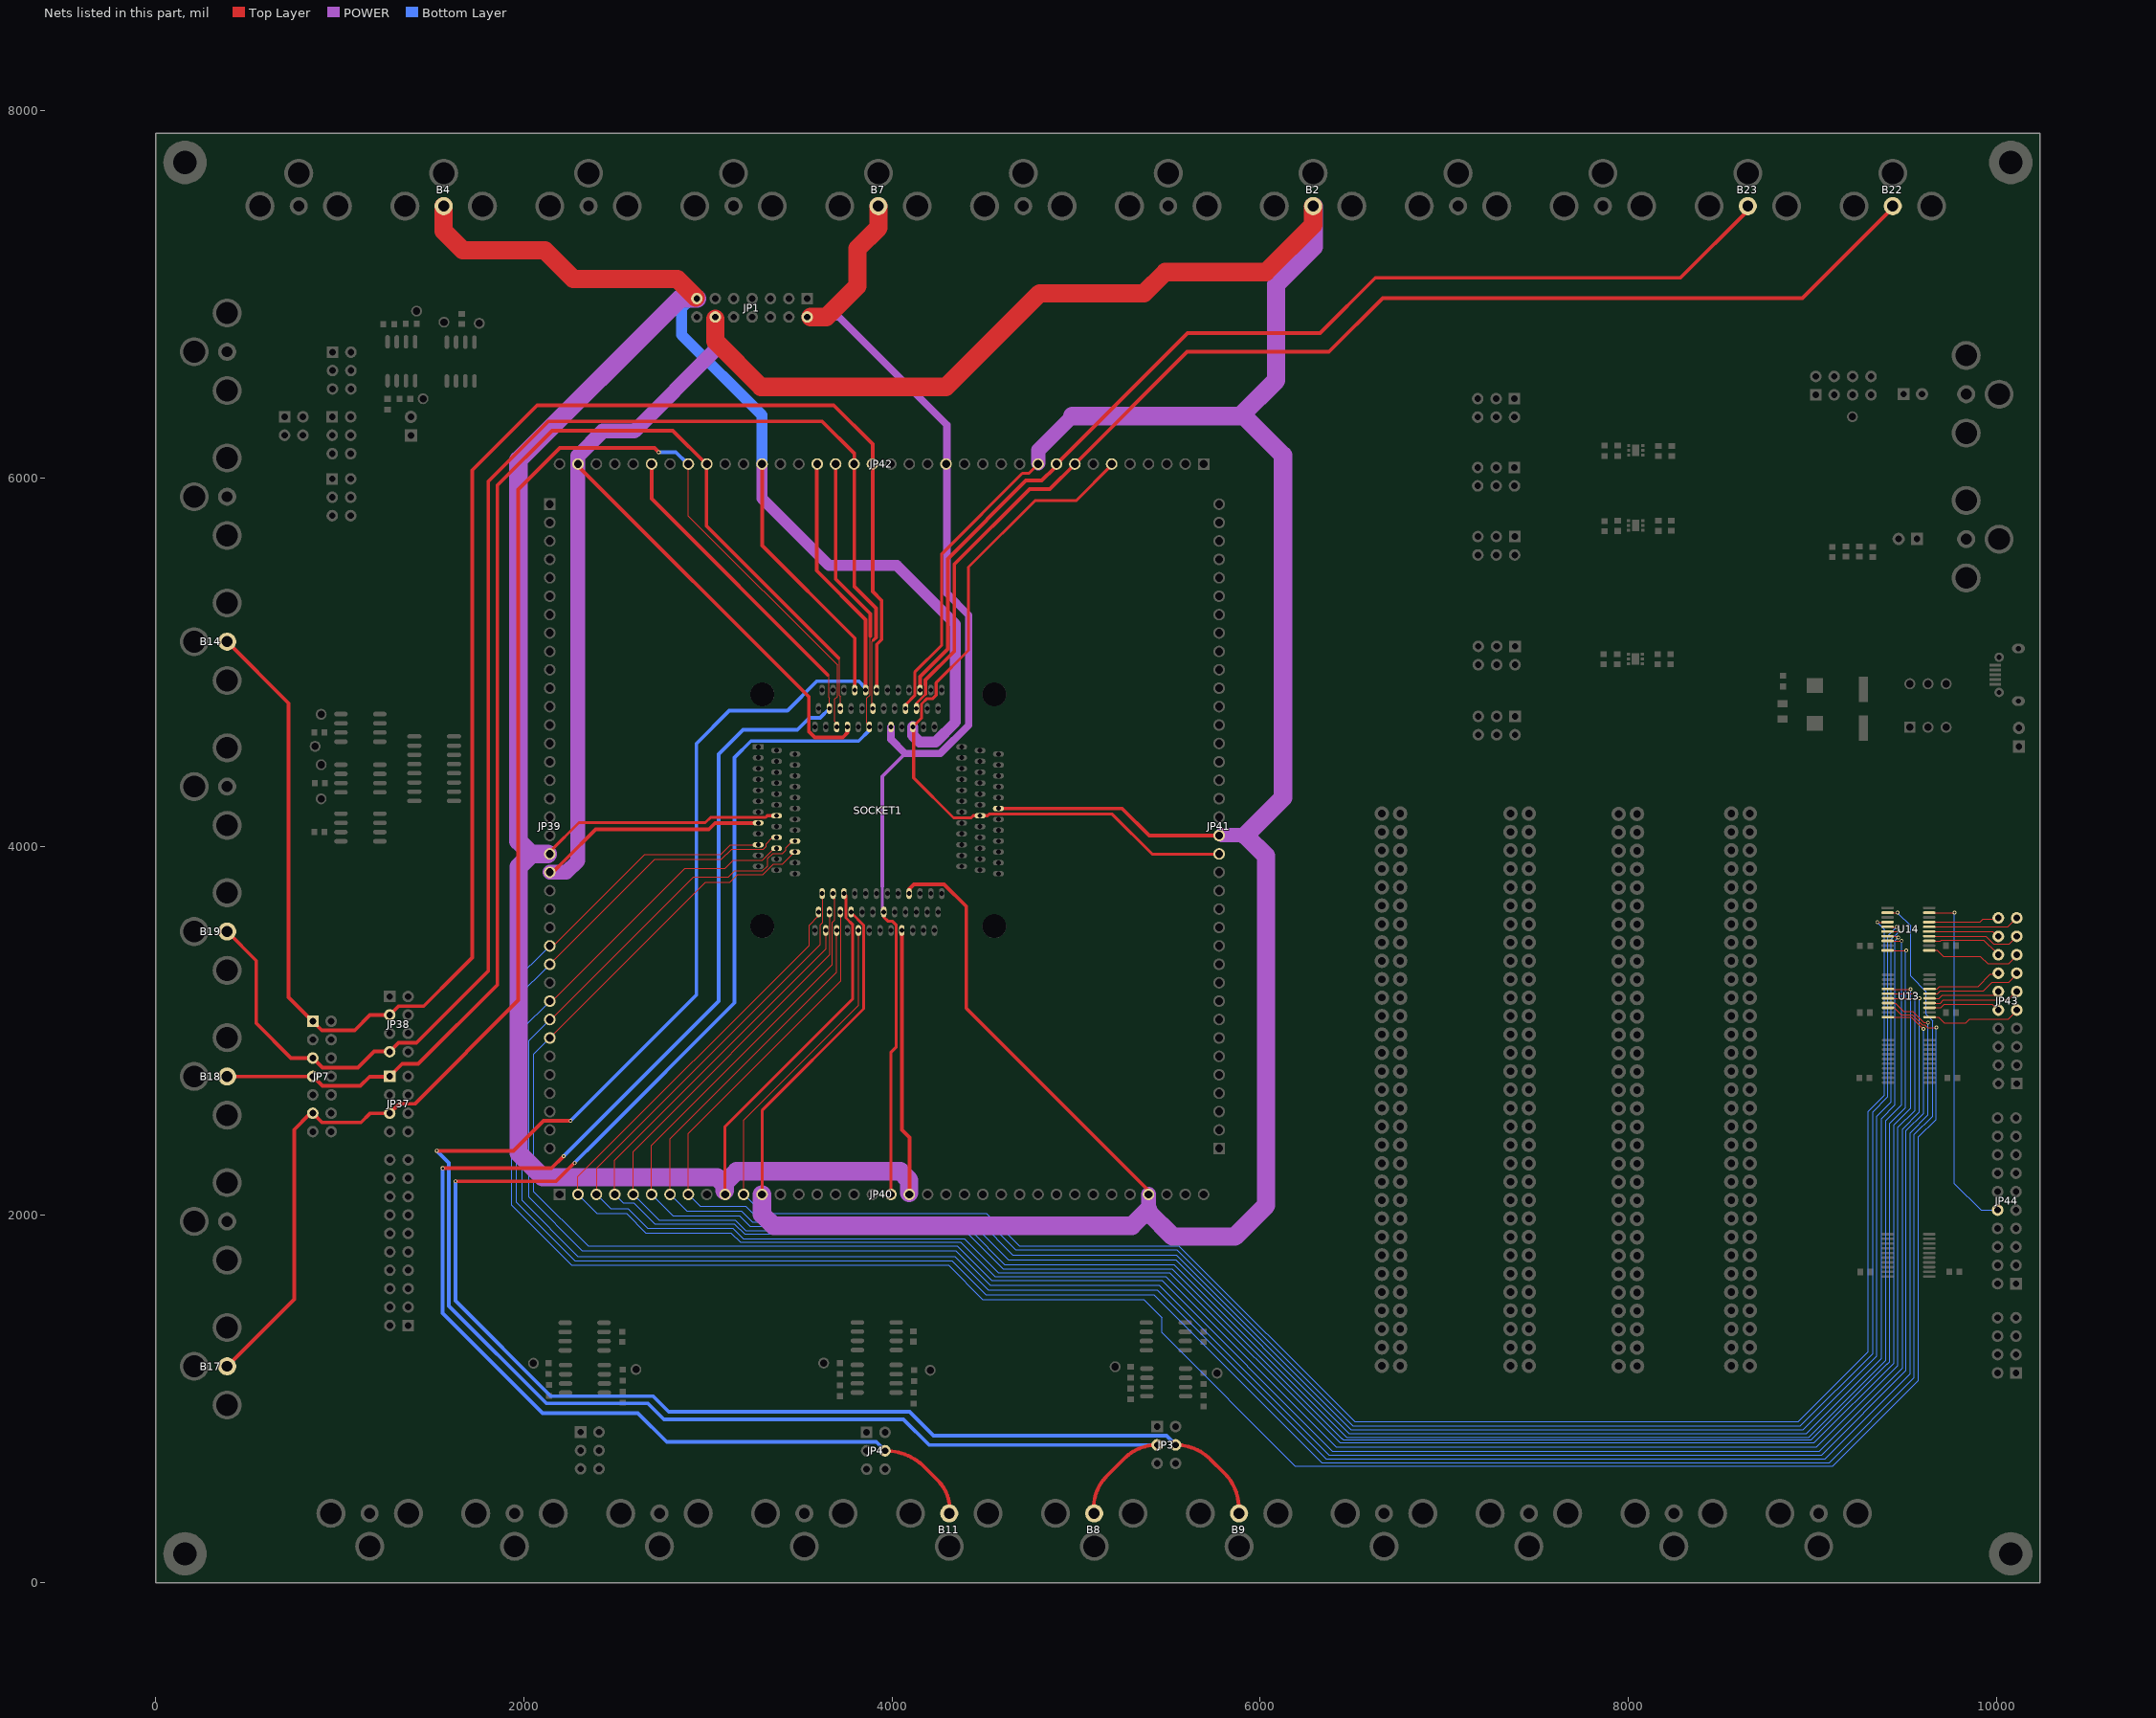
[diagram p0: the nets of this part, all layers, seen from the top]
# Altium PCB MISC62794.PcbDoc (part 6 of 7)
Units mil, origin at the board's own origin, x right, y up, seen from the top; angles counter-clockwise.
Board outline 10236.22 x 7874.02 mil, 4 copper layers (Top Layer, GND, POWER, Bottom Layer); 158 components, 185 nets, 1211 pads, 1759 vias.

## Via types
v1: diameter 20, hole 12, Top Layer to Bottom Layer, 1759 vias

## Nets (pads, with @x,y where several pads share a name; then routed paths per layer and width w, separated by ;. In a path a pad name is that pad's centre, name@x,y a point inside that pad or via, vN(x,y) a via of type N, cw(c..) or ccw(c..) an arc to the next point about the centre after c; other vN are vias at no path point) (continued)
VG2: B11.1 JP4.4 JP42.31 SOCKET1.140 | length 9670.1
  Top Layer w6: 3649.5,4934.5 3655.57,4928.43 3655.57,4809.69 3659.25,4806 SOCKET1.140@3659.25,4749.77
  Top Layer w20: v1(1558,2252) 2149,2252 v1(2215,2318) ; JP42.31@2693,6078.02 2693,5890 3649,4934 ; JP4.4@3961.48,717.38 cw(c3961.48,412.85) 4176.82,628.18 4246.12,558.88 cw(c4082.24,395) B11.1@4314,395
  Bottom Layer w20: v1(1558,2252) 1558,1464 2101,921 2619,921 2775.13,764.87 3913.98,764.87 JP4.4@3961.48,717.38 ; v1(2215,2318) 2371.5,2474.5 3057,3160 3057,4501 3190,4634 3485,4634 3550,4699 3608.48,4699 SOCKET1.140@3659.25,4749.77
VG_PS_CTRL: B17.1 JP7.11 JP37.5 JP42.29 SOCKET1.138 | length 8512
  Top Layer w6: JP42.29@2893,6058 2893,5796 3702.31,4986.69 3702.31,4815.31 3688,4801 3688,4679 SOCKET1.138@3696,4671
  Top Layer w20: B17.1@386.77,1176.09 751,1540.31 751,2462 JP7.11@835,2546 ; JP7.11@852,2551 902,2501 1114,2501 1163,2550 JP37.5@1253,2550 ; JP37.5@1269.93,2551.09 1320.83,2602 1406,2602 1969,3165 1969,5811 ; 1969,5822 1969,5811 ; v1(2732,6142) 2709,6165 2194,6165 1969,5940 1969,5811
  Bottom Layer w20: v1(2732,6142) 2825,6142 JP42.29@2885,6082
VG_PS_OUT: B22.1 JP42.8 SOCKET1.116 | length 6747.6
  Top Layer w12: SOCKET1.116@4131.69,4749.77 4131.69,4777.64 4183,4828.94
  Top Layer w16: 4182,4828 4182,4878.72
  Top Layer w20: 4181.28,4878.72 4181.28,4904.28 4338,5061 4338,5533 4747,5942 4856.98,5942 JP42.8@4993,6078.02 5602.98,6688 6374,6688 6666,6980 8947,6980 B22.1@9420,7453
VG_SEL<0>: JP40.4 SOCKET1.40 U14.20 | length 12002.8
  Top Layer w6: JP40.4@2493,2110.02 2493,2295 3642,3444 SOCKET1.40@3642,3534 ; U14.20@9431,3436 9432,3435 v1(9511,3435)
  Bottom Layer w6: JP40.4@2493,2110.02 2540.02,2063 2596,2063 2710,1949 3143,1949 3198,1894 4340,1894 ; 4363,1894 4340,1894 ; 4587,1721 4580,1728 ; 5504,1706 5487,1706 ; 6445,782 6431,796 ; 9408.5,1189.5 9390.5,1171.5 ; v1(9511,3435) 9506,3430 9506,2582 9420,2496 9420,1201 9390.5,1171.5 ; 4340,1894 4414,1894 4580,1728 ; 4580,1728 4602,1706 5487,1706 ; 5487,1706 5521,1706 6431,796 ; 6431,796 6451,776 8995,776 9390.5,1171.5
VG_SEL<0>_MCU: JP43.15 U14.1 | length 504.2
  Top Layer w6: U14.1@9635.03,3435.85 9679.15,3435.85 9711,3404 9913,3404 9954,3363 10068,3363 JP43.15@10097,3392
VG_SEL<1>: JP40.5 SOCKET1.41 U14.18 | length 11848.3
  Top Layer w6: JP40.5@2593,2110.02 2593,2343 3663,3413 SOCKET1.41@3663,3618 ; U14.18@9432,3487 v1(9486,3487)
  Bottom Layer w6: JP40.5@2593,2110.02 2733.02,1970 3148,1970 3205,1913 4428,1913 4612,1729 5532,1729 6470,791 8982,791 9399,1208 9399,2305 ; 9399,2308 9399,2305 ; v1(9486,3487) 9486,2598 9399,2511 9399,2305
VG_SEL<1>_MCU: JP43.16 U14.3 | length 391.4
  Top Layer w6: U14.3@9635.03,3487.03 9697.03,3487.03 9702,3492 9931,3492 JP43.16@9997,3426
VG_SEL<2>: JP40.6 SOCKET1.42 U14.17 | length 11785.9
  Top Layer w6: JP40.6@2693,2110.02 2693,2376 3675.25,3358.25 3675.25,3588.25 3688,3601 3688,3712 SOCKET1.42@3677,3723 ; U14.17@9427,3513 9460,3513 v1(9467,3506)
  Bottom Layer w6: JP40.6@2693,2110.02 2809.02,1994 3170,1994 3227,1937 4450,1937 4633,1754 5542,1754 6484,812 8968,812 9376,1220 9376,2523 9449,2596 9449,3488 v1(9467,3506)
VG_SEL<2>_MCU: JP43.17 U14.4 | length 486.1
  Top Layer w6: U14.4@9635.03,3512.62 9943.38,3512.62 9985,3471 10070,3471 JP43.17@10094,3495
VG_SEL<3>: JP40.7 SOCKET1.43 U14.16 | length 11455.5
  Top Layer w6: JP40.7@2793,2110.02 2793,2412 3699,3318 SOCKET1.43@3699,3532 ; U14.16@9430,3541 9432,3539 v1(9472,3539)
  Bottom Layer w6: JP40.7@2793,2110.02 2884.02,2019 3181,2019 3241,1959 4478,1959 4656,1781 5544,1781 6494,831 8949,831 9351,1233 9351,2296 ; 9351,2301 9351,2296 ; v1(9472,3539) 9429,3496 9429,2614 9351,2536 9351,2296
VG_SEL<3>_MCU: JP43.18 U14.5 | length 365.3
  Top Layer w6: U14.5@9635.03,3538.22 9978.78,3538.22 JP43.18@9994,3523
VG_SEL<4>: JP40.8 SOCKET1.44 U14.15 | length 11382.1
  Top Layer w6: JP40.8@2893,2110.02 2893,2441 3722,3270 SOCKET1.44@3722,3620 ; U14.15@9429,3563 v1(9458,3563)
  Bottom Layer w6: JP40.8@2893,2110.02 2958.02,2045 3205,2045 3267,1983 4497,1983 4671,1809 5546,1809 6503,852 8935,852 9329,1246 9329,2288 ; 9329,2297 9329,2288 ; v1(9458,3563) 9411,3516 9411,2744 9411,2641 9329,2559 9329,2288
VG_SEL<4>_MCU: JP43.19 U14.6 | length 476.1
  Top Layer w6: U14.6@9635.03,3563.81 10062.81,3563.81 JP43.19@10097,3598
VG_SEL<5>: JP40.11 SOCKET1.49 U14.14 | length 10920.2
  Top Layer w6: JP40.11@3194,2116 3194,2199 ; 3194,2162 3194,2199 ; SOCKET1.49@3816.73,3544.26 3816.73,3137.73 3194,2515 3194,2199 ; v1(9353,3589) U14.14@9384,3589
  Bottom Layer w6: JP40.11@3193,2110.02 3295.02,2008 4385,2008 4513,2008 4691,1830 5558,1830 6513,875 8923,875 9304,1256 9304,1687 9304,2561 9392,2649 9392,3550 v1(9353,3589)
VG_SEL<5>_MCU: JP43.20 U14.7 | length 364.8
  Top Layer w6: U14.7@9635.03,3589.4 9911.4,3589.4 9928,3606 JP43.20@9993,3606
VLIM: B14.1 JP7.1 JP38.3 JP42.19 SOCKET1.127 | length 9747.4
  Top Layer w6: SOCKET1.127@3915.16,4849.77 SOCKET1.127@3915.16,4861
  Top Layer w20: B14.1@386.77,5113.1 721,4778.87 721,3180 JP7.1@848,3053 ; JP7.1@852,3051 901,3002 1080,3002 1162,3084 JP38.3@1263,3084 ; JP38.3@1269.93,3085.09 1317.43,3132.59 1454.59,3132.59 1643,3321 ; 1659,3337 1643,3321 ; JP42.19@3894,6078.02 3894,6186 3683,6397 2071,6397 1719,6045 1719,3397 1643,3321 ; JP42.19@3895,6085 3895,5385 3943,5337 3943,5124 3917,5098 SOCKET1.127@3917,4861
VRES: B19.1 JP7.5 JP38.7 JP42.20 SOCKET1.128 | length 8412.5
  Top Layer w6: 3891.79,5108.79 3891.79,5105 ; SOCKET1.128@3895,4771 3891.79,4774.21 3891.79,5105 ; 3899,5121 3891.79,5113.79 3891.79,5105 ; 3900.5,5117.5 3901,5118
  Top Layer w20: B19.1@386.77,3538.29 545,3380.06 545,3040 734,2851 JP7.5@839,2851 ; JP7.5@852,2851 904,2799 1097,2799 1185,2887 JP38.7@1269,2887 ; JP38.7@1269.93,2885.09 1317.83,2933 1416,2933 1806,3323 1806,5984 2132,6310 3620,6310 3795,6135 3795,5412 3912,5295 3912,5135 3898.47,5121.47
VS1: B8.1 JP3.3 JP42.22 SOCKET1.130 | length 11127.6
  Top Layer w20: v1(1526,2347) 1943,2347 2106,2510 v1(2253,2510) ; JP42.22@3590,6067 3590,5499 3856.1,5232.9 SOCKET1.130@3856.1,4849.77 ; B8.1@5095,405 cw(c5346.08,405) 5168.54,582.54 5260.65,674.65 cw(c5440.19,495.11) JP3.3@5440.19,749.02
  Bottom Layer w20: v1@1527,2346 1592,2281 1592,1906 ; 1592,1936 1592,1906 ; v1(2253,2510) 2253,2511 2937,3195 2937,4560 3115,4738 3431,4738 3591,4898 3819,4898 3856.1,4860.9 SOCKET1.130@3856.1,4849.77 ; JP3.3@5440.19,749.02 4199.98,749.02 4062,887 2760,887 2672,975 2121,975 1592,1504 1592,1906
VS2: B9.1 JP3.4 JP42.21 SOCKET1.129 | length 10995.6
  Top Layer w6: SOCKET1.129@3872,4664 3863,4673 3863,4806 3879.47,4822.47 3879.47,5144
  Top Layer w20: v1(1628,2181) 2174,2181 2273,2280 v1(2275,2280) ; JP42.21@3693,6078.02 3693,5454 3882.1,5264.9 3882.1,5144 ; JP3.4@5540.19,749.02 cw(c5540.19,479.12) 5731.04,669.96 5805.51,595.49 cw(c5616.02,406) B9.1@5884,406
  Bottom Layer w20: 1627.06,1923.07 1627.06,1911 ; v1@1627.06,2181 1627.06,1911 ; v1(2275,2280) 2273,2280 2400,2407 3144,3151 3144,3188 3144,4484 3233,4573 3818,4573 3875.79,4630.79 SOCKET1.129@3875.79,4649.77 ; JP3.4@5540.19,749.02 5490.2,799 4224,799 4094,929 2786,929 2701,1014 2145,1014 1627.06,1531.94 1627.06,1911
VS_PS_CTRL: B18.1 JP7.7 JP37.1 JP42.28 SOCKET1.137 | length 7425.3
  Top Layer w6: 3710.5,5025.5 3714.31,5021.69 3714.31,4819.69 3718.31,4815.69 SOCKET1.137@3718.31,4749.77
  Top Layer w20: B18.1@386.77,2750.89 JP7.7@852.11,2750.89 ; JP7.7@852,2751 JP7.7@852.11,2750.89 ; JP7.7@857.89,2750.89 JP7.7@852.11,2750.89 ; JP37.1@1253,2749 1161,2749 1111,2699 904,2699 JP7.7@852.11,2750.89 ; JP37.1@1269.93,2751.09 1337.83,2819 1425,2819 1855,3249 1855,5775 ; 1855,5817 1855,5775 ; 3709,5024 2991,5742 2991,6077 2808,6260 2153,6260 1855,5962 1855,5775
VS_PS_OUT: B23.1 JP42.9 SOCKET1.115 | length 5917
  Top Layer w20: SOCKET1.115@4151.38,4849.77 4151.38,4923.38 4302,5074 4302,5563 4727,5988 4813,5988 JP42.9@4882,6057 ; JP42.9@4893,6078.02 5604.98,6790 6326,6790 6626,7090 8284,7090 B23.1@8649.84,7455.84 ; B23.1@8649.84,7479.17 B23.1@8649.84,7455.84 ; B23.1@8654,7460 B23.1@8649.84,7455.84
VS_SEL<0>: JP39.29 SOCKET1.27 U13.20 | length 13131.1
  Top Layer w6: JP39.29@2143,3067 2153,3067 2192,3106 ; 2181,3095 2192,3106 ; SOCKET1.27@3472.24,4029.69 3458.69,4029.69 3423,3994 3423,3981 3405,3963 3352,3963 3324,3935 3324,3895.45 3296.55,3868 3144,3868 3112,3836 2922,3836 2192,3106 ; U13.20@9442,3073 9537,3073 v1@9602,3008
  Bottom Layer w6: JP39.29@2140,3060.02 2026,2946.02 2026,2095 2316,1805 4346,1805 4533,1618 5452,1618 6375,695 9051,695 9510,1154 9510,2326 ; 9510,2333 9510,2326 ; v1@9602,3010 9605,3007 9605,2551 9510,2456 9510,2326
  other v1: 9604,3009
VS_SEL<0>_MCU: JP43.9 U13.1 | length 491.9
  Top Layer w6: U13.1@9637.03,3072.85 9685.15,3072.85 9717,3041 9833,3041 9854,3062 10066,3062 JP43.9@10095,3091
VS_SEL<1>: JP39.25 SOCKET1.28 U13.18 | length 13582.2
  Top Layer w6: JP39.25@2150,3450 2150,3451 2190,3491 ; 2183,3484 2190,3491 ; SOCKET1.28@3272.24,4010.01 3122.01,4010.01 3070,3958 2657,3958 2190,3491 ; U13.18@9410.97,3124.03 9444.97,3124.03 9482,3087 9542,3087 9597,3032 9611,3032 9626,3017 v1@9667,3017
  Bottom Layer w6: JP39.25@2140,3460.02 1934,3254.02 1934,2051 2259,1726 4306,1726 4492,1540 5367,1540 5466,1441 5466,1359 6190,635 9112,635 9577,1100 9577,2422 9672,2517 9672,3009 v1@9675,3012
  other v1: 9674,3017
VS_SEL<1>_MCU: JP43.10 U13.3 | length 381.8
  Top Layer w6: U13.3@9637.03,3124.03 9700.03,3124.03 9718,3142 9976,3142 JP43.10@10001,3117
VS_SEL<2>: JP39.28 SOCKET1.29 U13.17 | length 13255.7
  Top Layer w6: JP39.28@2138,3165 2157,3165 2181.5,3189.5 ; 2178,3186 2181.5,3189.5 ; SOCKET1.29@3372.24,3990.32 3361.32,3990.32 3296,3925 3136,3925 3092,3881 2873,3881 2181.5,3189.5 ; U13.17@9410.97,3149.62 9451.38,3149.62 9497,3104 9546,3104 9605,3045 9632,3045 v1@9635,3042
  Bottom Layer w6: JP39.28@2140,3160.02 1990,3010.02 1990,2076 2292,1774 4340,1774 4522,1592 5440,1592 6358,674 9071,674 9532,1135 9532,2445 9629,2542 v1@9629,3041
  other v1: 9629,3043
VS_SEL<2>_MCU: JP43.11 U13.4 | length 470.5
  Top Layer w6: U13.4@9637.03,3149.62 9695.62,3149.62 9713,3167 10065,3167 JP43.11@10090,3192
VS_SEL<3>: JP39.30 SOCKET1.30 U13.16 | length 13026.5
  Top Layer w6: JP39.30@2159,2975 2159,2980 2985,3806 3118,3806 3159,3847 3297,3847 3356,3906 3404,3906 3468.64,3970.64 SOCKET1.30@3472.24,3970.64 ; U13.16@9410.97,3175.22 v1(9582.78,3175.22)
  Bottom Layer w6: JP39.30@2140,2960.02 2053,2873.02 2053,2124 2348,1829 4354,1829 4541,1642 5466,1642 6392,716 9038,716 9490,1168 9490,2326 ; 9490,2327 9490,2326 ; v1(9582.78,3175.22) 9582.78,2557.78 9490,2465 9490,2326
VS_SEL<3>_MCU: JP43.12 U13.5 | length 375.3
  Top Layer w6: U13.5@9637.03,3175.22 9689.22,3175.22 9707,3193 9988,3193 JP43.12@10000,3205
VS_SEL<4>: JP40.2 SOCKET1.38 U13.15 | length 12178.8
  Top Layer w6: JP40.2@2293,2110.02 2293,2206 3549,3462 3549,3573 3600.2,3624.2 SOCKET1.38@3600.2,3644.26 ; U13.15@9437,3201 v1(9558,3201)
  Bottom Layer w6: JP40.2@2293,2110.02 2397.02,2006 2556,2006 2662,1900 3125,1900 3175,1850 4372,1850 4558,1664 5487,1664 6412,739 9024,739 9466,1181 9466,2475 9558,2567 v1(9558,3201)
VS_SEL<4>_MCU: JP43.13 U13.6 | length 501
  Top Layer w6: U13.6@9637.03,3200.81 9680.81,3200.81 9697,3217 9931,3217 9977,3263 10067,3263 JP43.13@10099,3295
VS_SEL<5>: JP40.3 SOCKET1.39 U13.14 | length 12087.9
  Top Layer w6: JP40.3@2395,2132 2395,2253 3610,3468 3610,3575 3623.57,3588.57 3623.57,3740.57 SOCKET1.39@3619.88,3744.26 ; U13.14@9427,3227 9429,3225 v1(9534,3225)
  Bottom Layer w6: JP40.3@2393,2110.02 2471.02,2032 2566,2032 2672,1926 3135,1926 3191,1870 4392,1870 4577,1685 5509,1685 6433,761 9011,761 9443,1193 9443,2489 9534,2580 v1(9534,3225)
VS_SEL<5>_MCU: JP43.14 U13.7 | length 396.9
  Top Layer w6: U13.7@9637.03,3226.4 9677.4,3226.4 9691,3240 9902,3240 9968,3306 JP43.14@9996,3306 ; JP43.14@9996,3310 JP43.14@10001,3310
VSS: B7.1 JP1.2 JP40.19 JP42.15 SOCKET1.56 SOCKET1.123 | length 6591.2
  Top Layer w16: SOCKET1.56@3954.53,3644.26 3954.53,3616.47 3976,3595 4000,3595 4023,3572 4023,2911 3993,2881 3993,2194 ; JP40.19@3993,2120 3993,2194 ; 3993,2159 3993,2194
  Top Layer w100: JP1.2@3558,6877 3643,6877 3812,7046 3812,7248 3925.43,7361.43 B7.1@3925.43,7479.17
  POWER w16: 3945.84,3782.84 3945.84,3652.95 SOCKET1.56@3954.53,3644.26
  POWER w20: 3945.84,3782.84 3945.84,4380.84 4063,4498
  POWER w40: JP1.2@3539,6877 3711,6877 4298,6290 4298,5375 4416,5257 4416,4659.8 4261.2,4505 4071,4505 3993.9,4582.1 SOCKET1.123@3993.9,4649.77
VSSC: B4.1 JP1.13 JP39.20 JP40.10 JP40.20 JP41.17 JP42.6 JP42.25 SOCKET1.20 SOCKET1.45 SOCKET1.61 SOCKET1.89 SOCKET1.117 SOCKET1.133 | length 23072.8
  Top Layer w16: JP39.20@2146,3978 2298,4130 2985,4130 3013.8,4158.8 3312.8,4158.8 3321.49,4167.49 SOCKET1.20@3372.24,4167.49 ; JP40.10@3091,2115 3091,2179 ; 3091,2159 3091,2179 ; SOCKET1.45@3737.99,3744.26 3748.99,3733.26 3748.99,3612.01 3786.05,3574.95 3786.05,3173.05 3091,2478 3091,2179 ; SOCKET1.117@4112.01,4649.77 4160.06,4697.83 4160.06,4774.37 4189.7,4804 4221,4804 4239,4822 4239,4890 4415,5066 4415,5518 4777,5880 5001,5880 JP42.6@5191,6070 ; SOCKET1.117@4117,4639 4117,4373 4333.92,4156.08 4350.44,4156.08 4350.85,4156.49 4404.66,4156.49 4405.08,4156.08 4429.08,4156.08 4440.49,4167.49 SOCKET1.89@4477.76,4167.49 4518.49,4167.49 4527.17,4176.17 5195.83,4176.17 5414,3958 JP41.17@5779,3958
  Top Layer w20: JP42.25@3294,6072 3294,5635 3797.05,5131.95 SOCKET1.133@3797.05,4849.77 ; SOCKET1.61@4052.95,3544.26 4052.95,2461.05 4094,2420 JP40.20@4094,2116
  Top Layer w80: JP1.13@2933,6983 JP1.13@2939,6977
  Top Layer w100: B4.1@1563.23,7479.17 1563.23,7343.77 1668,7239 2113,7239 2269,7083 2833,7083 JP1.13@2933,6983
  POWER w60: JP42.25@3293,6078.02 3293,5891 3657,5527 4025,5527 4344,5208 4344,4676 4236,4568 4149,4568 4112.01,4604.99 SOCKET1.117@4112.01,4649.77
  POWER w80: JP39.20@2128,3960 JP39.20@2133,3960 ; JP40.10@3092,2119 JP40.10@3092,2130 ; JP40.20@4093,2110.02 JP40.20@4093,2118
  POWER w100: 2040,3960 1970,4030 1970,6099 2848,6977 JP1.13@2939,6977 ; JP39.20@2128,3960 2042,3960 1971,3889 1971,2334 2102,2203 3048,2203 3090,2161 ; JP40.10@3090,2130 3090,2161 ; JP40.20@4092,2118 4092,2188 4044,2236 3155,2236 3090,2171 3090,2161
  Bottom Layer w60: JP1.13@2939,6977 2910,6977 2855,6922 2855,6781 3293,6343 JP42.25@3293,6078.02
VSSH: B2.1 JP1.12 JP39.21 JP40.12 JP40.33 JP41.18 JP42.10 JP42.35 SOCKET1.22 SOCKET1.47 SOCKET1.63 SOCKET1.91 SOCKET1.119 SOCKET1.135 | length 28436.7
  Top Layer w16: JP40.12@3295,2122 3295,2185 ; 3295,2172 3295,2185 ; SOCKET1.47@3777.36,3644.26 3777.36,3640.64 3845.1,3572.9 3845.1,3118.1 3295,2568 3295,2185 ; SOCKET1.119@4072.64,4749.77 4072.64,4769.64 4123.01,4820.01 4123.01,4947.01 4270,5094 4270,5590 4708,6028 4744,6028 JP42.10@4785,6069
  Top Layer w20: JP39.21@2151,3859 2155,3859 2224,3928 ; 2193,3897 2224,3928 ; JP42.35@2295,6079 2295,6065 3548,4812 3548,4624.18 3580.18,4592 3732,4592 3757.68,4617.68 SOCKET1.135@3757.68,4649.77 ; SOCKET1.22@3272.24,4128.12 3038.12,4128.12 3004,4094 2390,4094 2224,3928 ; SOCKET1.63@4092.32,3744.26 4092.32,3768.32 4118,3794 4283,3794 4403,3674 4403,3122 5347,2178 ; SOCKET1.91@4577.76,4206.86 5250.14,4206.86 5398,4059 5669,4059 ; 5370.41,2154.59 5347,2178 ; JP40.33@5399,2126 5347,2178 ; 5711,4059 5669,4059 ; JP41.18@5789,4059 5669,4059
  Top Layer w80: JP1.12@3040,6866 JP1.12@3040,6877 ; B2.1@6288,7479.17 B2.1@6288,7483
  Top Layer w100: JP1.12@3040,6866 3040,6745 3288,6497 4293,6497 4802,7006 5369,7006 5484,7121 6031,7121 6287.64,7377.64 B2.1@6287.64,7479.17
  POWER w40: JP39.21@2140,3860.02 JP39.21@2144,3860.02 ; JP1.12@3039,6871 JP1.12@3039,6877
  POWER w80: JP39.21@2140,3860.02 2229.02,3860.02 2292,3923 2292,6122 2427,6257 2599,6257 3037,6695 JP1.12@3037,6871 ; JP42.10@4794,6083 4794,6153 4979,6338 ; 5393,2034 JP40.33@5393,2110.02 ; JP41.18@5792,4062 5916,4062 ; B2.1@6287.64,7479 B2.1@6287.64,7479.17 ; B2.1@6289,7478 B2.1@6289,7479
  POWER w100: JP40.12@3293,2110.02 3293,2002 3356,1939 5303,1939 5391,2027 ; 4979,6338 5892,6338 6086,6532 6086,7054 6290,7258 B2.1@6290,7478 ; 5391,2015 5525,1881 5863,1881 6032,2050 6032,3949 5922,4059 ; 5911,6338 6124,6125 6124,4265 5918,4059
WL_TEST: JP39.26 SOCKET1.26 U14.12 | length 13937.6
  Top Layer w6: JP39.26@2154,3373 2154,3374 2710,3930 3073,3930 3129.64,3986.64 3299.64,3986.64 3315,4002 3315,4014 3350.38,4049.38 SOCKET1.26@3372.24,4049.38 ; U14.12@9428,3641 v1(9463,3641)
  Bottom Layer w6: JP39.26@2140,3360.02 1959,3179.02 1959,2068 2277,1750 4326,1750 4510,1566 5423,1566 6336,653 9093,653 9554,1114 9554,2335 ; v1(9463,3641) 9535,3569 9535,3296 9619,3212 9619,3088 9654,3053 9654,3017 ; 9554,2337 9554,2335 ; 9654,2982 9654,2978 ; 9654,3021 9654,3017 ; 9554,2335 9554,2435 9654,2535 9654,2978 ; 9654,2978 9654,3017
WL_TEST_MCU: JP44.10 U14.9 | length 1904
  Top Layer w6: U14.9@9635.03,3640.58 v1(9773.42,3640.58)
  Bottom Layer w6: v1@9773,3641 9773,2169 9916.99,2025.01 JP44.10@10007,2025.01
pads on no net: IC1.7 IC1.9 IC2.5 IC3.5 IC4.5 JP6.5 JP6.6 JP11.17 JP11.18 JP11.19 JP11.20 JP39.1 JP39.2 JP39.3 JP39.4 JP39.5 JP39.6 JP39.31 JP39.32 JP39.33 JP39.34 JP39.35 JP39.36 JP40.1 JP40.36 JP41.1 JP41.2 JP41.3 JP41.4 JP41.5 JP41.6 JP41.31 JP41.32 JP41.33 JP41.34 JP41.35 JP41.36 JP42.1 JP42.36 JP44.12 JP44.13 JP44.14 JP44.15 JP44.16 JP44.17 JP44.18 JP44.19 JP44.20 S1.3 S1.4 SOCKET1. SOCKET1.1 SOCKET1.2 SOCKET1.3 SOCKET1.4 SOCKET1.5 SOCKET1.6 SOCKET1.31 SOCKET1.32 SOCKET1.33 SOCKET1.34 SOCKET1.35 SOCKET1.36 SOCKET1.37 SOCKET1.72 SOCKET1.73 SOCKET1.74 SOCKET1.75 SOCKET1.76 SOCKET1.77 SOCKET1.78 SOCKET1.103 SOCKET1.104 SOCKET1.105 SOCKET1.106 SOCKET1.107 SOCKET1.108 SOCKET1.109 SOCKET1.144 SP1.1 SP2.1 SP3.1 SP4.1 U15.9 U15.12 USB1.2 USB1.3 USB1.4

## Polygon pours and split planes (outlines as drawn)
NetB25_1 on Top Layer "Bottom Layer-No Net" (solid, remove dead copper, pour order 1000): 9561,6462 9561,6432 9561,6385 9570,6376 9586,6360 9614,6360 9870,6360 9877,6367 9886,6376 9886,6453 9886,6517 9866,6537 9862,6541 9802,6541 9580,6541 9568,6529 9561,6522 9561,6463
DCDC_OUT on Top Layer "Bottom Layer-No Net" (solid, remove dead copper, pour order 1001): 9286,6466 9286,6375 9298,6363 9320,6341 9378,6341 9519,6341 9528,6350 9533,6355 9533,6434 9533,6495 9526,6502 9521,6507 9489,6507 9301,6507 9292,6498 9286,6492 9286,6469
USB_5V on Top Layer "Bottom Layer-No Net" (solid, remove dead copper, pour order 1002): 8829,6458 8829,5689 8859,5659 8905,5613 9343,5613 9485,5613 9499,5627 9506,5634 9506,5695 9506,5843 9484,5865 9480,5869 9427,5869 9215,5869 9185,5899 9151,5933 9151,6445 9151,6478 9146,6483 9139,6490 9069,6490 8861,6490 8829,6458
3V3 on Top Layer "Bottom Layer-No Net" (solid, remove dead copper, pour order 1003): 6846,4894 6846,4876 6846,4556 6862,4540 6898,4504 7076,4504 7295,4504 7310,4519 7315,4524 7315,4581 7315,4625 7307,4633 7302,4638 7289,4638 7081,4638 7072,4647 7056,4663 7056,4717 7056,4894 7073,4911 7076,4914 7145,4914 7297,4914 7309,4926 7315,4932 7315,4976 7315,5006 7303,5018 7301,5020 7270,5020 7076,5020 7059,5037 7053,5043 7053,5103 7053,5143 7082,5172 7093,5183 7239,5183 7708,5183 7727,5164 7750,5141 7750,5105 7750,5063 7770,5043 7785,5028 7882,5028 7968,5028 7971,5031 7976,5036 7989,5036 8005,5036 8007,5038 8009,5040 8009,5276 7961,5324 7916,5369 7340,5369 6916,5369 6865,5318 6846,5299 6846,4895
V11 on Top Layer "Bottom Layer-No Net" (solid, remove dead copper, pour order 1004): 6825,5719 6825,5547 6840,5532 6858,5514 6941,5514 7195,5514 7212,5531 7218,5537 7218,5582 7218,5597 7205,5610 7201,5614 7169,5614 7067,5614 7049,5632 7030,5651 7030,5696 7030,5858 7056,5884 7060,5888 7115,5888 7207,5888 7218,5899 7218,5965 7218,5979 7206,5991 7188,5991 7053,5991 7039,6005 7034,6010 7034,6059 7034,6200 7062,6228 7072,6238 7142,6238 7189,6238 7203,6252 7224,6273 7224,6313 7224,6357 7211,6370 7204,6377 7174,6377 7080,6377 7061,6396 7046,6411 7046,6445 7046,6506 7082,6542 7110,6570 7316,6570 7496,6570 7535,6531 7588,6478 7588,6318 7588,6200 7604,6184 7626,6162 7931,6162 7968,6162 7974,6168 7975,6169 7998,6169 8008,6169 8010,6171 8011,6172 8011,6175 8011,6836 7947,6900 7940,6907 7705,6907 6992,6907 6933,6848 6825,6740 6825,5721
V25 on Top Layer "Bottom Layer-No Net" (solid, remove dead copper, pour order 1005): 7246,5585 7246,5444 7258,5432 7275,5415 7304,5415 7724,5415 7736,5427 7769,5460 7769,5587 7769,5713 7790,5734 7808,5752 7885,5752 7959,5752 7966,5759 7969,5762 7997,5762 8009,5762 8011,5764 8011,5770 8011,5894 8002,5903 7996,5909 7995,5910 7790,5910 7740,5910 7717,5933 7707,5943 7707,6023 7707,6100 7682,6125 7669,6138 7643,6138 7616,6138 7557,6197 7502,6252 7427,6252 7359,6252 7335,6276 7325,6286 7325,6329 7325,6350 7313,6362 7307,6368 7290,6368 7259,6368 7252,6361 7246,6355 7246,6340 7246,6198 7269,6175 7302,6142 7347,6142 7418,6142 7420,6142 7526,6036 7526,5988 7526,5931 7502,5907 7477,5882 7415,5882 7349,5882 7335,5896 7320,5911 7320,5954 7320,5980 7311,5989 7304,5996 7295,5996 7258,5996 7252,5990 7244,5982 7244,5964 7244,5823 7270,5797 7287,5780 7352,5780 7435,5780 7459,5756 7480,5735 7480,5701 7480,5549 7465,5534 7456,5525 7424,5525 7351,5525 7345,5531 7325,5551 7325,5583 7325,5600 7314,5611 7308,5617 7288,5617 7262,5617 7252,5607 7246,5601 7246,5585
VCC_5V on Top Layer "Bottom Layer-No Net" (solid, remove dead copper, pour order 1006): 221 vertices, not listed, extent 7346,4350 9890,6278
NetJP32_1 on Top Layer "Bottom Layer-No Net" (solid, remove dead copper, pour order 1007): 9590,4643 9590,4467 9603,4454 9634,4423 9687,4423 10156,4423 10170,4437 10172,4439 10172,4462 10172,4562 10157,4577 10150,4584 10119,4584 9680,4584 9664,4600 9664,4637 9664,4668 9656,4676 9651,4681 9632,4681 9605,4681 9595,4671 9590,4666 9590,4643
NetS1_5 on Top Layer "Bottom Layer-No Net" (solid, remove dead copper, pour order 1008): 9590,4915 9590,4868 9599,4859 9605,4853 9628,4853 9651,4853 9660,4862 9664,4866 9664,4898 9664,4914 9679,4929 9693,4943 9739,4943 9764,4943 9803,4904 9859,4848 9916,4848 9954,4848 9974,4868 9979,4873 9991,4873 10026,4873 10027,4874 10028,4875 10028,4878 10028,4888 10027,4889 10026,4890 10023,4890 9954,4890 9940,4904 9815,5029 9695,5029 9618,5029 9597,5008 9590,5001 9590,4916
GND on Top Layer "Bottom Layer-No Net" (solid, remove dead copper, pour order 1009): -343,7235 -343,-190 -96,-437 264,-797 1052,-797 10434,-797 10704,-527 10839,-392 10839,-347 10839,8001 10322,8518 10052,8788 9534,8788 129,8788 -141,8518 -366,8293 -366,7280
VCC_5V on Bottom Layer "Bottom Layer-No Net" (solid, remove dead copper, pour order 1010): 7355,4988 7355,4922 7390,4887 7406,4871 7474,4871 7595,4871 7712,4754 7771,4695 8009,4695 8041,4695 8072,4726 8081,4735 8081,4823 8081,4829 8048,4862 7864,4862 7820,4906 7793,4933 7793,5014 7793,6293 7721,6365 7719,6367 7416,6367 7364,6367 7352,6355 7349,6352 7349,6336 7349,6272 7365,6256 7387,6234 7480,6234 7491,6234 7513,6212 7545,6180 7545,6110 7545,6029 7529,6013 7508,5992 7394,5992 7365,5992 7353,5980 7348,5975 7348,5961 7348,5910 7362,5896 7371,5887 7405,5887 7507,5887 7534,5860 7548,5846 7548,5807 7548,5661 7527,5640 7505,5618 7399,5618 7367,5618 7356,5607 7351,5602 7351,5582 7351,5546 7361,5536 7372,5525 7399,5525 7498,5525 7526,5497 7534,5489 7534,5469 7534,5070 7515,5051 7486,5022 7403,5022 7374,5022 7361,5009 7355,5003 7355,4989
GND on Bottom Layer "Bottom Layer-No Net" (solid, remove dead copper, pour order 1011): -1008,7549 -1008,-233 -515,-726 -104,-1137 417,-1137 10335,-1137 10856,-616 11267,-205 11267,1877 11267,8315 10609,8973 10143,9439 8335,9439 6,9439 -487,8946 -1008,8425 -1008,7658
GND on POWER "Bottom Layer-No Net" (solid, remove dead copper, pour order 1012): -501,7348 -501,-235 -96,-640 16,-752 917,-752 10232,-752 10524,-460 10592,-392 10592,-325 10592,8000 10209,8383 9939,8653 9714,8653 152,8653 -186,8315 -456,8045 -456,7505
GND on GND (split plane): 10216.12,20.1 20.1,20.1 20.1,7853.92 10216.12,7853.92

## Keep-outs
Keep-Out Layer:
  the board outline again, w5